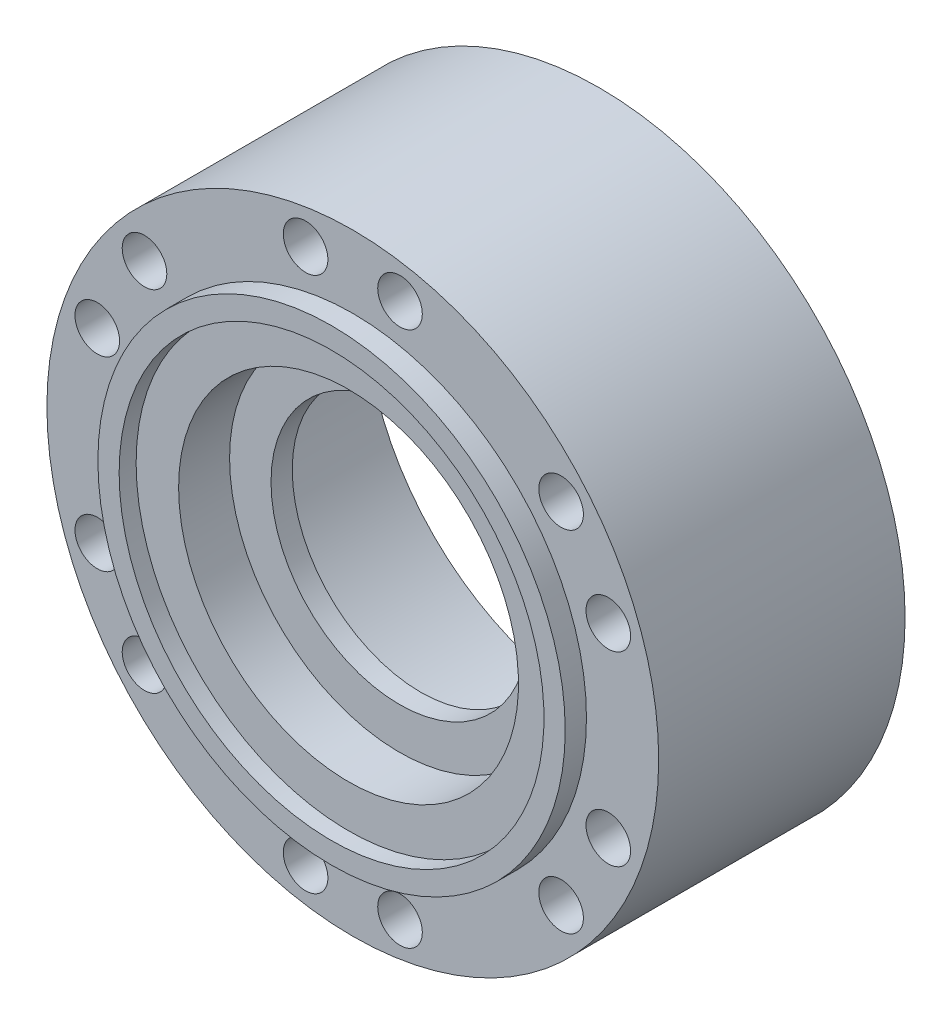
SolidWorks part; units mm, degrees
material "普通碳钢"
ref_plane "Front Plane" through (0, 0, 0) normal (0, 0, 1) x (1, 0, 0)
ref_plane "Top Plane" through (0, 0, 0) normal (0, 1, 0) x (1, 0, 0)
ref_plane "Right Plane" through (0, 0, 0) normal (1, 0, 0) x (0, 0, -1)
sketch "Sketch1" plane through (0, 0, 0) normal (0, 0, 1) x (1, 0, 0)
  circle A0 centre (0, 0) radius 72
  dimension "D1" = 144
extrude "Boss-Extrude1" add sketch "Sketch1" along normal blind 58
sketch "Sketch2" plane through (0, 0, 58) normal (0, 0, 1) x (1, 0, 0)
  circle A0 centre (0, 0) radius 55
  dimension "D1" = 110
extrude "Boss-Extrude2" add sketch "Sketch2" along normal blind 5
hole_wizard "Ø10.5 (10.5) Diameter Hole1" positions "Sketch4" profile "Sketch3" hole size "Ø10.5" standard "GB" end condition through all
sketch "Sketch4" plane through (0, 0, 0) normal (0, 0, -1) x (-1, 0, 0)
  line L0 (0, 0) -> (12.0425, 68.2966) construction
  line L3 (0, 0) -> (-12.2163, 69.2821) construction
  line L5 (0, 0) -> (0, 96.0771) construction
  circle A1 centre (0, 0) radius 64 construction
  point P0 (-11.1135, 63.0277)
  point P33 (11.1135, 63.0277)
  point P41 (49.0268, 41.1384)
  point P42 (60.1403, 21.8893)
  point P43 (60.1403, -21.8893)
  point P44 (49.0268, -41.1384)
  point P45 (11.1135, -63.0277)
  point P46 (-11.1135, -63.0277)
  point P47 (-49.0268, -41.1384)
  point P48 (-60.1403, -21.8893)
  point P49 (-60.1403, 21.8893)
  point P50 (-49.0268, 41.1384)
  dimension "D1" = 128
  dimension "D2" = 10
  dimension "D3" = 10
  dimension "D4" = 6
sketch "Sketch3" plane through (11.1135, 63.0277, 0) normal (1, 0, 0) x (0, 1, 0)
  line L0 (0, 0) -> (0, 63)
  line L1 (0, 63) -> (5.25, 63)
  line L2 (5.25, 63) -> (5.25, 0)
  line L5 (5.25, 0) -> (0, 0)
  line L11 (0, -6.35) -> (0, 107.95) construction
  dimension "通孔孔直径" = 10.5
  dimension "通孔孔深度" = 63
sketch "Sketch5" plane through (0, 0, 0) normal (0, 0, -1) x (-1, 0, 0)
  circle A0 centre (0, 0) radius 55
  dimension "D1" = 110
extrude "Cut-Extrude1" cut sketch "Sketch5" against normal blind 42
sketch "Sketch6" plane through (0, 0, 42) normal (0, 0, -1) x (-1, 0, 0)
  circle A0 centre (0, 0) radius 30.25
  dimension "D1" = 60.5
extrude "Cut-Extrude2" cut sketch "Sketch6" against normal blind 5
sketch "Sketch7" plane through (0, 0, 47) normal (0, 0, -1) x (-1, 0, 0)
  circle A0 centre (0, 0) radius 40
  dimension "D1" = 80
extrude "Cut-Extrude3" cut sketch "Sketch7" against normal blind 12
sketch "Sketch9" plane through (0, 0, 59) normal (0, 0, -1) x (-1, 0, 0)
  circle A0 centre (0, 0) radius 50
  dimension "D1" = 100
extrude "Cut-Extrude4" cut sketch "Sketch9" against normal blind 4
